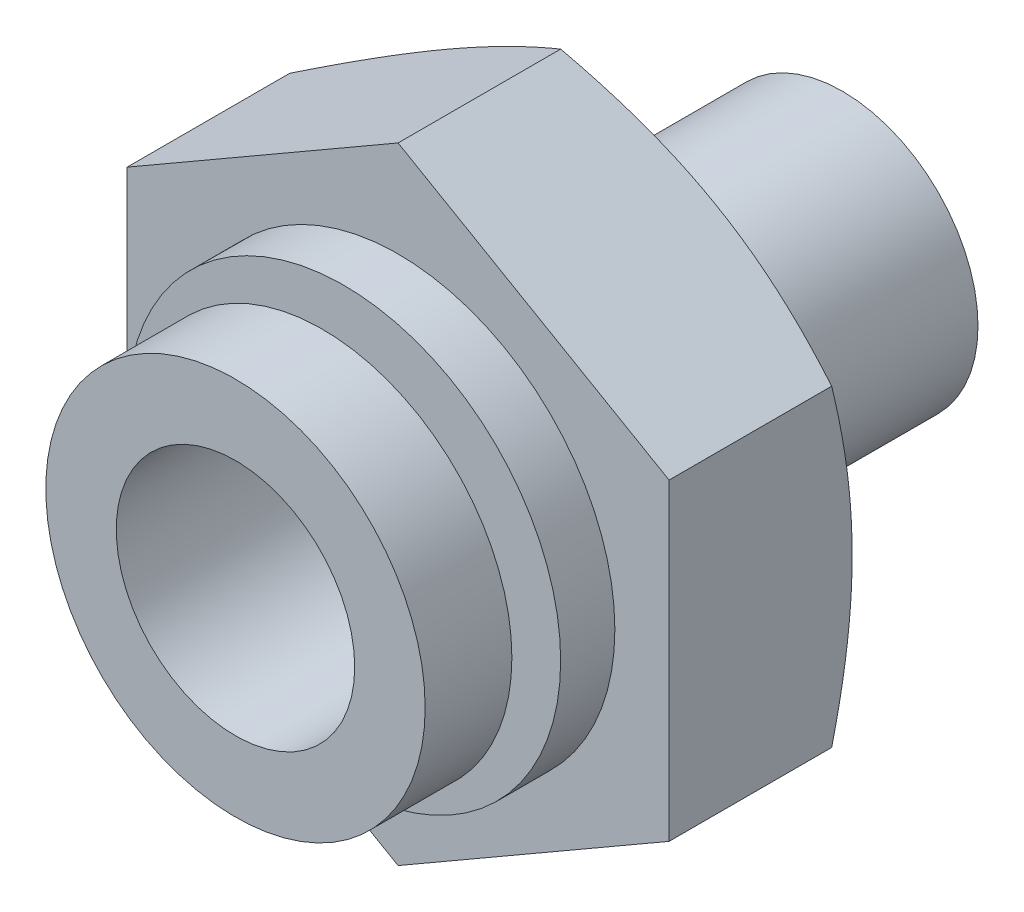
SolidWorks part; units mm, degrees
ref_plane "Front Plane" through (0, 0, 0) normal (0, 0, 1) x (1, 0, 0)
ref_plane "Top Plane" through (0, 0, 0) normal (0, 1, 0) x (1, 0, 0)
ref_plane "Right Plane" through (0, 0, 0) normal (1, 0, 0) x (0, 0, -1)
sketch "Sketch1" plane through (0, 0, 0) normal (0, 0, 1) x (1, 0, 0)
  line L1 (0, 28.8675) -> (-25, 14.4338)
  line L2 (-25, 14.4338) -> (-25, -14.4338)
  line L3 (-25, -14.4338) -> (0, -28.8675)
  line L4 (0, -28.8675) -> (25, -14.4338)
  line L5 (25, -14.4338) -> (25, 14.4338)
  line L6 (25, 14.4338) -> (0, 28.8675)
  circle A0 centre (0, 0) radius 25 construction
  dimension "D1" = 50
extrude "Boss-Extrude1" add sketch "Sketch1" along normal mid plane 23
sketch "Sketch3" plane through (0, 0, 0) normal (1, 0, 0) x (0, 0, -1)
  line L0 (-1000, 0) -> (49000, 0) construction
  line L1 (11.5, 12.5) -> (3.5, 28.8675)
  line L2 (11.5, -14.4338) -> (11.5, 14.4338) construction
  line L3 (-11.5, 28.8675) -> (11.5, 28.8675) construction
  line L4 (3.5, 28.8675) -> (11.5, 28.8675)
  line L5 (11.5, 28.8675) -> (11.5, 12.5)
  dimension "D1" = 8
  dimension "D2" = 12.5
revolve "Cut-Revolve1" cut sketch "Sketch3" angle 360 about L0
sketch "Sketch4" plane through (0, 0, -11.5) normal (0, 0, -1) x (-1, 0, 0)
  circle A0 centre (0, 0) radius 12.5
  dimension "D1" = 25
extrude "Boss-Extrude2" add sketch "Sketch4" along normal blind 18
sketch "Sketch5" plane through (0, 0, 11.5) normal (0, 0, 1) x (1, 0, 0)
  circle A0 centre (0, 0) radius 20
  dimension "D1" = 40
extrude "Boss-Extrude3" add sketch "Sketch5" along normal blind 5
sketch "Sketch6" plane through (0, 0, 16.5) normal (0, 0, 1) x (1, 0, 0)
  circle A0 centre (0, 0) radius 14
  dimension "D1" = 28
extrude "Boss-Extrude4" add sketch "Sketch6" along normal blind 2
sketch "Sketch7" plane through (0, 0, 18.5) normal (0, 0, 1) x (1, 0, 0)
  circle A0 centre (0, 0) radius 17.5
  dimension "D1" = 35
extrude "Boss-Extrude5" add sketch "Sketch7" along normal blind 8
sketch "Sketch8" plane through (0, 0, 26.5) normal (0, 0, 1) x (1, 0, 0)
  circle A0 centre (0, 0) radius 11
  dimension "D1" = 22
extrude "Cut-Extrude1" cut sketch "Sketch8" against normal blind 28
sketch "Sketch9" plane through (0, 0, -29.5) normal (0, 0, -1) x (-1, 0, 0)
  circle A0 centre (0, 0) radius 10
  dimension "D1" = 20
extrude "Cut-Extrude2" cut sketch "Sketch9" against normal blind 71
